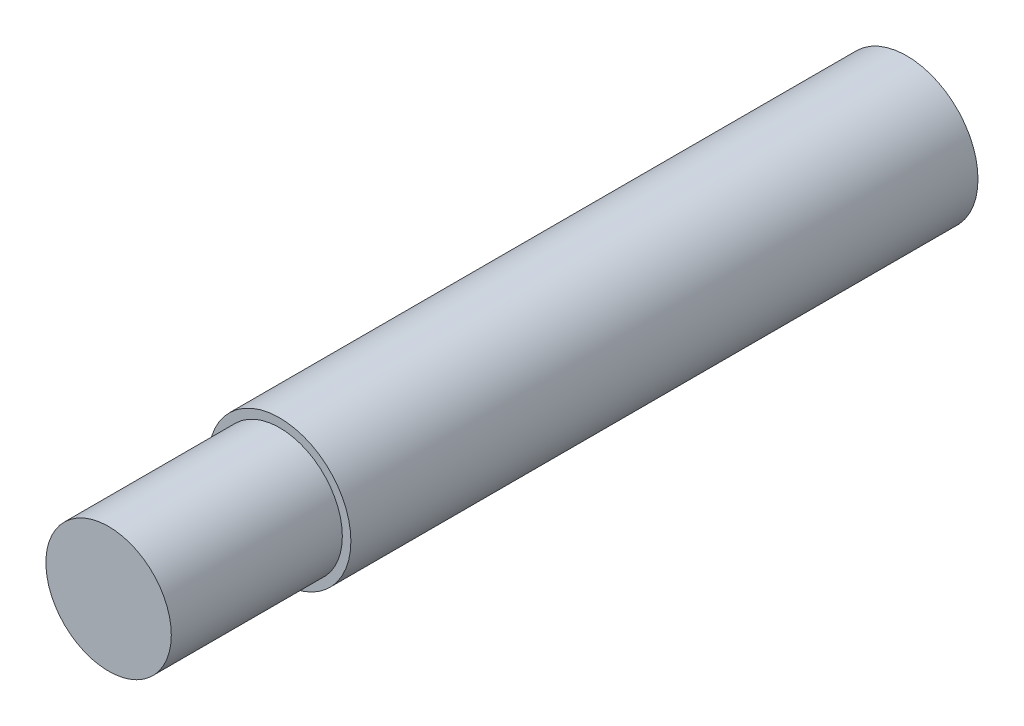
from build123d import *

# Parameters (mm, degrees)
SKETCH_1_R      = 1.25
EXTRUDE_1_DEPTH = 11
SKETCH_2_R      = 1.1
EXTRUDE_2_DEPTH = 3


with BuildPart() as part:
    # 草图1 → 凸台-拉伸1 (new body)
    with BuildSketch(Plane.XY):
        Circle(SKETCH_1_R)
    extrude(amount=EXTRUDE_1_DEPTH)

    # 草图2 → 凸台-拉伸2 (add)
    with BuildSketch(Plane.XY.offset(11)):
        Circle(SKETCH_2_R)
    extrude(amount=EXTRUDE_2_DEPTH)


solid = part.part
